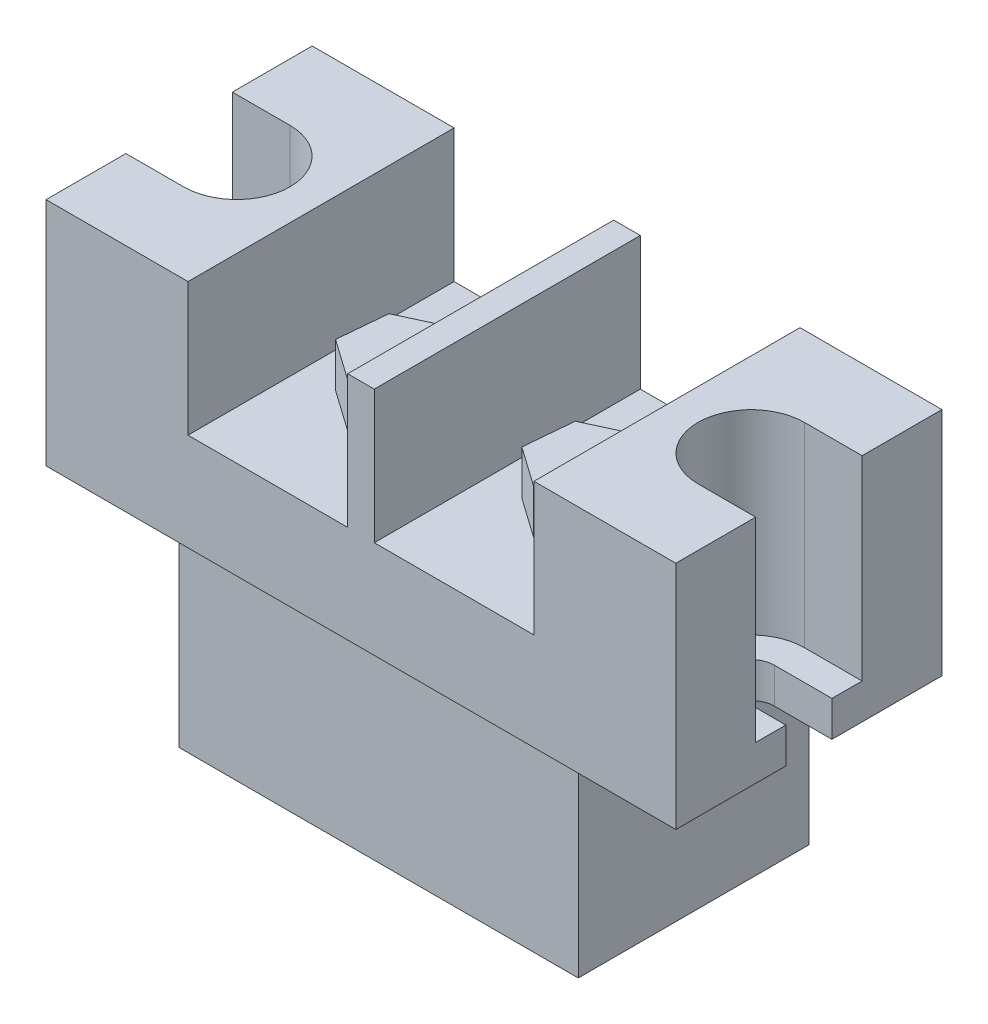
from build123d import *

# Parameters (mm, degrees)
SKETCH_1_W             = 71
SKETCH_1_H             = 30
EXTRUDE_1_DEPTH        = 26
SKETCH_2_W             = 45
SKETCH_2_H             = 26
EXTRUDE_2_DEPTH        = 22
CUT_EXTRUDE_1_DEPTH    = 62.556884262
CUT_EXTRUDE_2_DEPTH    = 22
SKETCH_5_W             = 18
SKETCH_5_H             = 30
CUT_EXTRUDE_3_DEPTH    = 15
PATTERN_LINEAR_1_COUNT = 2
PATTERN_LINEAR_1_PITCH = 21
EXTRUDE_3_DEPTH        = 5
PATTERN_LINEAR_2_COUNT = 2
PATTERN_LINEAR_2_PITCH = 21


with BuildPart() as part:
    # 草图1 → 凸台-拉伸1 (new body)
    with BuildSketch(Plane(origin=(0, 0, 0), x_dir=(1, 0, 0), z_dir=(0, 1, 0))):
        Rectangle(SKETCH_1_W, SKETCH_1_H)
    extrude(amount=EXTRUDE_1_DEPTH)

    # 草图2 → 凸台-拉伸2 (add)
    with BuildSketch(Plane.XZ):
        Rectangle(SKETCH_2_W, SKETCH_2_H)
    extrude(amount=EXTRUDE_2_DEPTH)

    # 草图3 → 切除-拉伸1 (cut, through all)
    with BuildSketch(Plane(origin=(0, 26, 0), x_dir=(1, 0, 0), z_dir=(0, 1, 0))):
        with BuildLine():
            Line((-29, -2.6), (-61.70015948, -2.6))
            ThreePointArc((-61.70015948, -2.6), (-64.30015948, 0), (-61.70015948, 2.6))
            Line((-61.70015948, 2.6), (-29, 2.6))
            ThreePointArc((-29, 2.6), (-26.4, 0), (-29, -2.6))
        make_face()
        with BuildLine():
            Line((29, 2.6), (61.70015948, 2.6))
            ThreePointArc((61.70015948, 2.6), (64.30015948, 0), (61.70015948, -2.6))
            Line((61.70015948, -2.6), (29, -2.6))
            ThreePointArc((29, -2.6), (26.4, 0), (29, 2.6))
        make_face()
    extrude(amount=-CUT_EXTRUDE_1_DEPTH, mode=Mode.SUBTRACT)

    # 草图4 → 切除-拉伸2 (cut)
    with BuildSketch(Plane(origin=(0, 26, 0), x_dir=(1, 0, 0), z_dir=(0, 1, 0))):
        with BuildLine():
            Line((29, 6), (52.513840992, 6))
            ThreePointArc((52.513840992, 6), (58.513840992, 0), (52.513840992, -6))
            Line((52.513840992, -6), (29, -6))
            ThreePointArc((29, -6), (23, 0), (29, 6))
        make_face()
        with BuildLine():
            Line((-29, -6), (-53.007180335, -6))
            ThreePointArc((-53.007180335, -6), (-59.007180335, 0), (-53.007180335, 6))
            Line((-53.007180335, 6), (-29, 6))
            ThreePointArc((-29, 6), (-23, 0), (-29, -6))
        make_face()
    extrude(amount=-CUT_EXTRUDE_2_DEPTH, mode=Mode.SUBTRACT)

    # 草图5 → 切除-拉伸3 (cut)
    with BuildSketch(Plane(origin=(0, 26, 0), x_dir=(1, 0, 0), z_dir=(0, 1, 0))):
        with Locations((10.5, 0)):
            Rectangle(SKETCH_5_W, SKETCH_5_H)
    cut_extrude_3 = extrude(amount=-CUT_EXTRUDE_3_DEPTH, mode=Mode.SUBTRACT)

    # 阵列(线性)1: 切除-拉伸3 ×2
    with Locations(*[(-i * PATTERN_LINEAR_1_PITCH, 0, 0) for i in range(1, PATTERN_LINEAR_1_COUNT)]):
        add(cut_extrude_3, mode=Mode.SUBTRACT)

    # 草图6 → 凸台-拉伸3 (add)
    with BuildSketch(Plane(origin=(0, 11, 0), x_dir=(1, 0, 0), z_dir=(0, 1, 0))):
        Polygon((15.033036482, -3.195715708), (15.534089227, 2.327866896), (11.001052745, 5.523582603), (5.966963518, 3.195715708), (5.465910773, -2.327866896), (9.998947255, -5.523582603), align=None)
    extrude_3 = extrude(amount=EXTRUDE_3_DEPTH)

    # 阵列(线性)2: 凸台-拉伸3 ×2
    with Locations(*[(-i * PATTERN_LINEAR_2_PITCH, 0, 0) for i in range(1, PATTERN_LINEAR_2_COUNT)]):
        add(extrude_3)


solid = part.part
